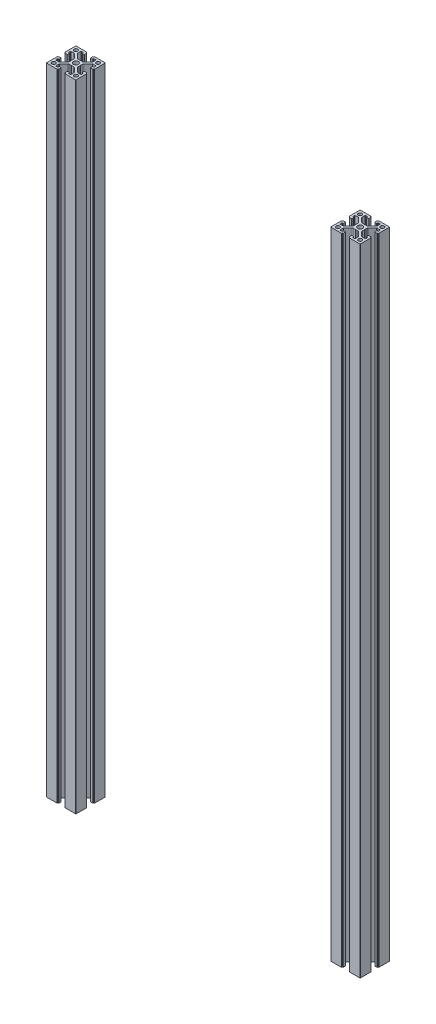
SolidWorks part; units mm, degrees
material "6061 合金"
ref_plane "前视基准面" through (0, 0, 0) normal (0, 0, 1) x (1, 0, 0)
ref_plane "上视基准面" through (0, 0, 0) normal (0, 1, 0) x (1, 0, 0)
ref_plane "右视基准面" through (0, 0, 0) normal (1, 0, 0) x (0, 0, -1)
sketch "草图1" plane through (0, 0, 0) normal (0, 0, 1) x (1, 0, 0)
  line L0 (192.5, 0) -> (-192.5, 0) construction
  line L1 (-192.5, 0) -> (-192.5, 861)
  line L2 (-212.5, 861) -> (212.5, 861)
  line L4 (0, 861) -> (0, 0) construction
  line L5 (-192.5, 80) -> (192.5, 80)
  line L8 (192.5, 0) -> (192.5, 861)
  dimension "D1" = 20
  dimension "D2" = 425
  dimension "D3" = 861
  dimension "D4" = 80
other "LE-8-5050W"
ref_plane "基准面4" through (-192.5, 0, 0) normal (0, 1, 0) x (-1, 0, 0)
sketch "草图14" plane through (-192.5, 0, 0) normal (0, 1, 0) x (-1, 0, 0)
  line L0 (-6, -0.3) -> (-6, -3.0503)
  line L1 (-6.5858, -4.4645) -> (-12.2249, -10.1036)
  line L2 (-12.5784, -10.25) -> (-16.8, -10.25)
  line L3 (-17.3, -9.75) -> (-17.3, -7.6)
  line L4 (-16.8, -7.1) -> (-16, -7.1)
  line L5 (-15.5, -6.6) -> (-15.5, -4.6)
  line L6 (-16, -4.1) -> (-18.7, -4.1)
  line L7 (-19, -4.4) -> (-19, -4.8)
  line L8 (-19.3, -5.1) -> (-19.7, -5.1)
  line L9 (-20, -5.4) -> (-20, -19.5)
  line L10 (-19.5, -20) -> (-5.4, -20)
  line L11 (-5.1, -19.7) -> (-5.1, -19.3)
  line L12 (-4.8, -19) -> (-4.4, -19)
  line L13 (-4.1, -18.7) -> (-4.1, -16)
  line L14 (-4.6, -15.5) -> (-6.6, -15.5)
  line L15 (-7.1, -16) -> (-7.1, -16.8)
  line L16 (-7.6, -17.3) -> (-9.75, -17.3)
  line L17 (-10.25, -16.8) -> (-10.25, -12.5784)
  line L18 (-10.1036, -12.2249) -> (-4.4645, -6.5858)
  line L19 (-3.0503, -6) -> (-0.3, -6)
  line L20 (0.3, -6) -> (3.0503, -6)
  line L21 (4.4645, -6.5858) -> (10.1036, -12.2249)
  line L22 (10.25, -12.5784) -> (10.25, -16.8)
  line L23 (9.75, -17.3) -> (7.6, -17.3)
  line L24 (7.1, -16.8) -> (7.1, -16)
  line L25 (6.6, -15.5) -> (4.6, -15.5)
  line L26 (4.1, -16) -> (4.1, -18.7)
  line L27 (4.4, -19) -> (4.8, -19)
  line L28 (5.1, -19.3) -> (5.1, -19.7)
  line L29 (5.4, -20) -> (19.5, -20)
  line L30 (20, -19.5) -> (20, -5.4)
  line L31 (19.7, -5.1) -> (19.3, -5.1)
  line L32 (19, -4.8) -> (19, -4.4)
  line L33 (18.7, -4.1) -> (16, -4.1)
  line L34 (15.5, -4.6) -> (15.5, -6.6)
  line L35 (16, -7.1) -> (16.8, -7.1)
  line L36 (17.3, -7.6) -> (17.3, -9.75)
  line L37 (16.8, -10.25) -> (12.5784, -10.25)
  line L38 (12.2249, -10.1036) -> (6.5858, -4.4645)
  line L39 (6, -3.0503) -> (6, -0.3)
  line L40 (6, 0.3) -> (6, 3.0503)
  line L41 (6.5858, 4.4645) -> (12.2249, 10.1036)
  line L42 (12.5784, 10.25) -> (16.8, 10.25)
  line L43 (17.3, 9.75) -> (17.3, 7.6)
  line L44 (16.8, 7.1) -> (16, 7.1)
  line L45 (15.5, 6.6) -> (15.5, 4.6)
  line L46 (16, 4.1) -> (18.7, 4.1)
  line L47 (19, 4.4) -> (19, 4.8)
  line L48 (19.3, 5.1) -> (19.7, 5.1)
  line L49 (20, 5.4) -> (20, 19.5)
  line L50 (19.5, 20) -> (5.4, 20)
  line L51 (5.1, 19.7) -> (5.1, 19.3)
  line L52 (4.8, 19) -> (4.4, 19)
  line L53 (4.1, 18.7) -> (4.1, 16)
  line L54 (4.6, 15.5) -> (6.6, 15.5)
  line L55 (7.1, 16) -> (7.1, 16.8)
  line L56 (7.6, 17.3) -> (9.75, 17.3)
  line L57 (10.25, 16.8) -> (10.25, 12.5784)
  line L58 (10.1036, 12.2249) -> (4.4645, 6.5858)
  line L59 (3.0503, 6) -> (0.3, 6)
  line L60 (-0.3, 6) -> (-3.0503, 6)
  line L61 (-4.4645, 6.5858) -> (-10.1036, 12.2249)
  line L62 (-10.25, 12.5784) -> (-10.25, 16.8)
  line L63 (-9.75, 17.3) -> (-7.6, 17.3)
  line L64 (-7.1, 16.8) -> (-7.1, 16)
  line L65 (-6.6, 15.5) -> (-4.6, 15.5)
  line L66 (-4.1, 16) -> (-4.1, 18.7)
  line L67 (-4.4, 19) -> (-4.8, 19)
  line L68 (-5.1, 19.3) -> (-5.1, 19.7)
  line L69 (-5.4, 20) -> (-19.5, 20)
  line L70 (-20, 19.5) -> (-20, 5.4)
  line L71 (-19.7, 5.1) -> (-19.3, 5.1)
  line L72 (-19, 4.8) -> (-19, 4.4)
  line L73 (-18.7, 4.1) -> (-16, 4.1)
  line L74 (-15.5, 4.6) -> (-15.5, 6.6)
  line L75 (-16, 7.1) -> (-16.8, 7.1)
  line L76 (-17.3, 7.6) -> (-17.3, 9.75)
  line L77 (-16.8, 10.25) -> (-12.5784, 10.25)
  line L78 (-12.2249, 10.1036) -> (-6.5858, 4.4645)
  line L79 (-6, 3.0503) -> (-6, 0.3)
  circle A0 centre (-15, 15) radius 2.45
  circle A1 centre (0, 0) radius 3.4
  circle A2 centre (15, 15) radius 2.45
  circle A3 centre (15, -15) radius 2.45
  circle A4 centre (-15, -15) radius 2.45
  arc A5 (-6, -0.3) -> (-6, 0.3) centre (-6, 0) ccw
  arc A6 (-6.5858, -4.4645) -> (-6, -3.0503) centre (-8, -3.0503) ccw
  arc A7 (-12.5784, -10.25) -> (-12.2249, -10.1036) centre (-12.5784, -9.75) ccw
  arc A8 (-17.3, -9.75) -> (-16.8, -10.25) centre (-16.8, -9.75) ccw
  arc A9 (-16.8, -7.1) -> (-17.3, -7.6) centre (-16.8, -7.6) ccw
  arc A10 (-16, -7.1) -> (-15.5, -6.6) centre (-16, -6.6) ccw
  arc A11 (-15.5, -4.6) -> (-16, -4.1) centre (-16, -4.6) ccw
  arc A12 (-18.7, -4.1) -> (-19, -4.4) centre (-18.7, -4.4) ccw
  arc A13 (-19.3, -5.1) -> (-19, -4.8) centre (-19.3, -4.8) ccw
  arc A14 (-19.7, -5.1) -> (-20, -5.4) centre (-19.7, -5.4) ccw
  arc A15 (-20, -19.5) -> (-19.5, -20) centre (-19.5, -19.5) ccw
  arc A16 (-5.4, -20) -> (-5.1, -19.7) centre (-5.4, -19.7) ccw
  arc A17 (-4.8, -19) -> (-5.1, -19.3) centre (-4.8, -19.3) ccw
  arc A18 (-4.4, -19) -> (-4.1, -18.7) centre (-4.4, -18.7) ccw
  arc A19 (-4.1, -16) -> (-4.6, -15.5) centre (-4.6, -16) ccw
  arc A20 (-6.6, -15.5) -> (-7.1, -16) centre (-6.6, -16) ccw
  arc A21 (-7.6, -17.3) -> (-7.1, -16.8) centre (-7.6, -16.8) ccw
  arc A22 (-10.25, -16.8) -> (-9.75, -17.3) centre (-9.75, -16.8) ccw
  arc A23 (-10.1036, -12.2249) -> (-10.25, -12.5784) centre (-9.75, -12.5784) ccw
  arc A24 (-3.0503, -6) -> (-4.4645, -6.5858) centre (-3.0503, -8) ccw
  arc A25 (0.3, -6) -> (-0.3, -6) centre (0, -6) ccw
  arc A26 (4.4645, -6.5858) -> (3.0503, -6) centre (3.0503, -8) ccw
  arc A27 (10.25, -12.5784) -> (10.1036, -12.2249) centre (9.75, -12.5784) ccw
  arc A28 (9.75, -17.3) -> (10.25, -16.8) centre (9.75, -16.8) ccw
  arc A29 (7.1, -16.8) -> (7.6, -17.3) centre (7.6, -16.8) ccw
  arc A30 (7.1, -16) -> (6.6, -15.5) centre (6.6, -16) ccw
  arc A31 (4.6, -15.5) -> (4.1, -16) centre (4.6, -16) ccw
  arc A32 (4.1, -18.7) -> (4.4, -19) centre (4.4, -18.7) ccw
  arc A33 (5.1, -19.3) -> (4.8, -19) centre (4.8, -19.3) ccw
  arc A34 (5.1, -19.7) -> (5.4, -20) centre (5.4, -19.7) ccw
  arc A35 (19.5, -20) -> (20, -19.5) centre (19.5, -19.5) ccw
  arc A36 (20, -5.4) -> (19.7, -5.1) centre (19.7, -5.4) ccw
  arc A37 (19, -4.8) -> (19.3, -5.1) centre (19.3, -4.8) ccw
  arc A38 (19, -4.4) -> (18.7, -4.1) centre (18.7, -4.4) ccw
  arc A39 (16, -4.1) -> (15.5, -4.6) centre (16, -4.6) ccw
  arc A40 (15.5, -6.6) -> (16, -7.1) centre (16, -6.6) ccw
  arc A41 (17.3, -7.6) -> (16.8, -7.1) centre (16.8, -7.6) ccw
  arc A42 (16.8, -10.25) -> (17.3, -9.75) centre (16.8, -9.75) ccw
  arc A43 (12.2249, -10.1036) -> (12.5784, -10.25) centre (12.5784, -9.75) ccw
  arc A44 (6, -3.0503) -> (6.5858, -4.4645) centre (8, -3.0503) ccw
  arc A45 (6, 0.3) -> (6, -0.3) centre (6, 0) ccw
  arc A46 (6.5858, 4.4645) -> (6, 3.0503) centre (8, 3.0503) ccw
  arc A47 (12.5784, 10.25) -> (12.2249, 10.1036) centre (12.5784, 9.75) ccw
  arc A48 (17.3, 9.75) -> (16.8, 10.25) centre (16.8, 9.75) ccw
  arc A49 (16.8, 7.1) -> (17.3, 7.6) centre (16.8, 7.6) ccw
  arc A50 (16, 7.1) -> (15.5, 6.6) centre (16, 6.6) ccw
  arc A51 (15.5, 4.6) -> (16, 4.1) centre (16, 4.6) ccw
  arc A52 (18.7, 4.1) -> (19, 4.4) centre (18.7, 4.4) ccw
  arc A53 (19.3, 5.1) -> (19, 4.8) centre (19.3, 4.8) ccw
  arc A54 (19.7, 5.1) -> (20, 5.4) centre (19.7, 5.4) ccw
  arc A55 (20, 19.5) -> (19.5, 20) centre (19.5, 19.5) ccw
  arc A56 (5.4, 20) -> (5.1, 19.7) centre (5.4, 19.7) ccw
  arc A57 (4.8, 19) -> (5.1, 19.3) centre (4.8, 19.3) ccw
  arc A58 (4.4, 19) -> (4.1, 18.7) centre (4.4, 18.7) ccw
  arc A59 (4.1, 16) -> (4.6, 15.5) centre (4.6, 16) ccw
  arc A60 (6.6, 15.5) -> (7.1, 16) centre (6.6, 16) ccw
  arc A61 (7.6, 17.3) -> (7.1, 16.8) centre (7.6, 16.8) ccw
  arc A62 (10.25, 16.8) -> (9.75, 17.3) centre (9.75, 16.8) ccw
  arc A63 (10.1036, 12.2249) -> (10.25, 12.5784) centre (9.75, 12.5784) ccw
  arc A64 (3.0503, 6) -> (4.4645, 6.5858) centre (3.0503, 8) ccw
  arc A65 (-0.3, 6) -> (0.3, 6) centre (0, 6) ccw
  arc A66 (-4.4645, 6.5858) -> (-3.0503, 6) centre (-3.0503, 8) ccw
  arc A67 (-10.25, 12.5784) -> (-10.1036, 12.2249) centre (-9.75, 12.5784) ccw
  arc A68 (-9.75, 17.3) -> (-10.25, 16.8) centre (-9.75, 16.8) ccw
  arc A69 (-7.1, 16.8) -> (-7.6, 17.3) centre (-7.6, 16.8) ccw
  arc A70 (-7.1, 16) -> (-6.6, 15.5) centre (-6.6, 16) ccw
  arc A71 (-4.6, 15.5) -> (-4.1, 16) centre (-4.6, 16) ccw
  arc A72 (-4.1, 18.7) -> (-4.4, 19) centre (-4.4, 18.7) ccw
  arc A73 (-5.1, 19.3) -> (-4.8, 19) centre (-4.8, 19.3) ccw
  arc A74 (-5.1, 19.7) -> (-5.4, 20) centre (-5.4, 19.7) ccw
  arc A75 (-19.5, 20) -> (-20, 19.5) centre (-19.5, 19.5) ccw
  arc A76 (-20, 5.4) -> (-19.7, 5.1) centre (-19.7, 5.4) ccw
  arc A77 (-19, 4.8) -> (-19.3, 5.1) centre (-19.3, 4.8) ccw
  arc A78 (-19, 4.4) -> (-18.7, 4.1) centre (-18.7, 4.4) ccw
  arc A79 (-16, 4.1) -> (-15.5, 4.6) centre (-16, 4.6) ccw
  arc A80 (-15.5, 6.6) -> (-16, 7.1) centre (-16, 6.6) ccw
  arc A81 (-17.3, 7.6) -> (-16.8, 7.1) centre (-16.8, 7.6) ccw
  arc A82 (-16.8, 10.25) -> (-17.3, 9.75) centre (-16.8, 9.75) ccw
  arc A83 (-12.2249, 10.1036) -> (-12.5784, 10.25) centre (-12.5784, 9.75) ccw
  arc A84 (-6, 3.0503) -> (-6.5858, 4.4645) centre (-8, 3.0503) ccw
  point P250 (0, 0)
sketch "草图15" plane through (0, 861, 0) normal (0, 1, 0) x (1, 0, 0)
  line L0 (-192.5, 0) -> (192.5, 0) construction
sketch "草图16" plane through (0, 861, 0) normal (0, 1, 0) x (1, 0, 0)
  point P0 (0, 0)
